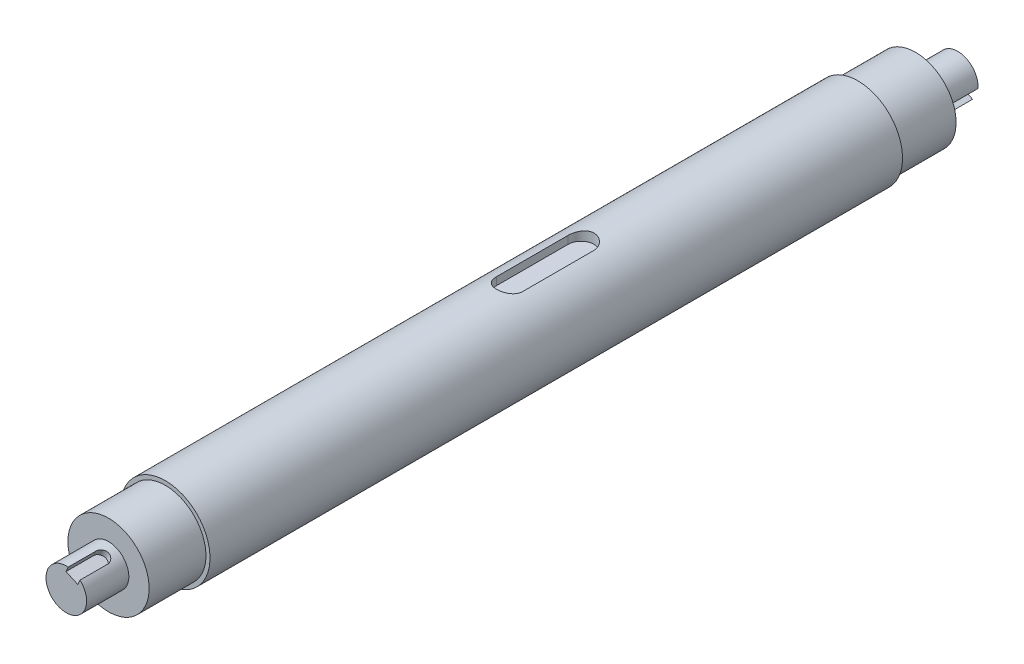
SolidWorks part; units mm, degrees
ref_plane "前视基准面" through (0, 0, 0) normal (0, 0, 1) x (1, 0, 0)
ref_plane "上视基准面" through (0, 0, 0) normal (0, 1, 0) x (1, 0, 0)
ref_plane "右视基准面" through (0, 0, 0) normal (1, 0, 0) x (0, 0, -1)
sketch "草图1" plane through (0, 0, 0) normal (0, 1, 0) x (1, 0, 0)
  line L0 (0, 0) -> (0, -80836.6018) construction
  line L1 (0, 100) -> (-12.5, 100)
  line L2 (-12.5, 100) -> (-12.5, 74)
  line L3 (-12.5, 74) -> (-25, 74)
  line L4 (-25, 74) -> (-25, 38.53)
  line L5 (-25, 38.53) -> (-27.5, 38.53)
  line L6 (-27.5, 38.53) -> (-27.5, -387.93)
  line L7 (-27.5, -387.93) -> (-25, -387.93)
  line L8 (-25, -387.93) -> (-25, -422.93)
  line L9 (-25, -422.93) -> (-12.5, -422.93)
  line L10 (-12.5, -422.93) -> (-12.5, -448.93)
  line L11 (-12.5, -448.93) -> (0, -448.93)
  line L12 (0, -448.93) -> (0, 100)
  dimension "D1" = 25
  dimension "D2" = 26
  dimension "D3" = 35.47
  dimension "D4" = 55
  dimension "D5" = 50
  dimension "D6" = 100
  dimension "D7" = 35
  dimension "D8" = 26
  dimension "D9" = 426.46
revolve "旋转1" add sketch "草图1" angle 360 about L0
ref_plane "基准面3" through (0, 0, 174.465) normal (0, 0, -1) x (-1, 0, 0)
ref_plane "基准面4" through (0, 27.5, 0) normal (0, 1, 0) x (1, 0, 0)
sketch "草图6" plane through (0, 27.5, 0) normal (0, 1, 0) x (1, 0, 0)
  line L0 (0, -131.93) -> (0, -175.93) construction
  line L1 (8, -131.93) -> (8, -175.93)
  line L2 (-8, -131.93) -> (-8, -175.93)
  line L3 (-12.5, -448.93) -> (12.5, -448.93) construction
  arc A0 (8, -131.93) -> (-8, -131.93) centre (0, -131.93) ccw
  arc A1 (-8, -175.93) -> (8, -175.93) centre (0, -175.93) ccw
  point P2 (0, -153.93)
  dimension "D2" = 265
  dimension "D3" = 44
  dimension "D1" = 16
extrude "切除-拉伸3" cut sketch "草图6" against normal blind 6
sketch "草图7" plane through (14.434, -6.4264, 0) normal (-0.9135, 0.4067, 0) x (0, 0, 1)
  line L0 (-105.8478, 0) -> (-83, 0) construction
  line L1 (-105.8478, 4) -> (-83, 4)
  line L2 (-105.8478, -4) -> (-83, -4)
  line L3 (-74, 12.5) -> (-74, -12.5) construction
  arc A0 (-105.8478, 4) -> (-105.8478, -4) centre (-105.8478, 0) ccw
  arc A1 (-83, -4) -> (-83, 4) centre (-83, 0) ccw
  point P2 (-94.4239, 0)
  dimension "D2" = 5
  dimension "D1" = 8
extrude "切除-拉伸4" cut sketch "草图7" along normal blind 7.3
sketch "草图8" plane through (6.4264, 14.434, 0) normal (-0.4067, -0.9135, 0) x (0, 0, 1)
  line L0 (455.3039, 0) -> (431.93, 0) construction
  line L1 (455.3039, -4) -> (431.93, -4)
  line L2 (455.3039, 4) -> (431.93, 4)
  line L3 (422.93, -12.5) -> (422.93, 12.5) construction
  arc A0 (455.3039, -4) -> (455.3039, 4) centre (455.3039, 0) ccw
  arc A1 (431.93, 4) -> (431.93, -4) centre (431.93, 0) ccw
  point P3 (443.617, 0)
  dimension "D2" = 5
  dimension "D1" = 8
extrude "切除-拉伸5" cut sketch "草图8" along normal blind 7.3
